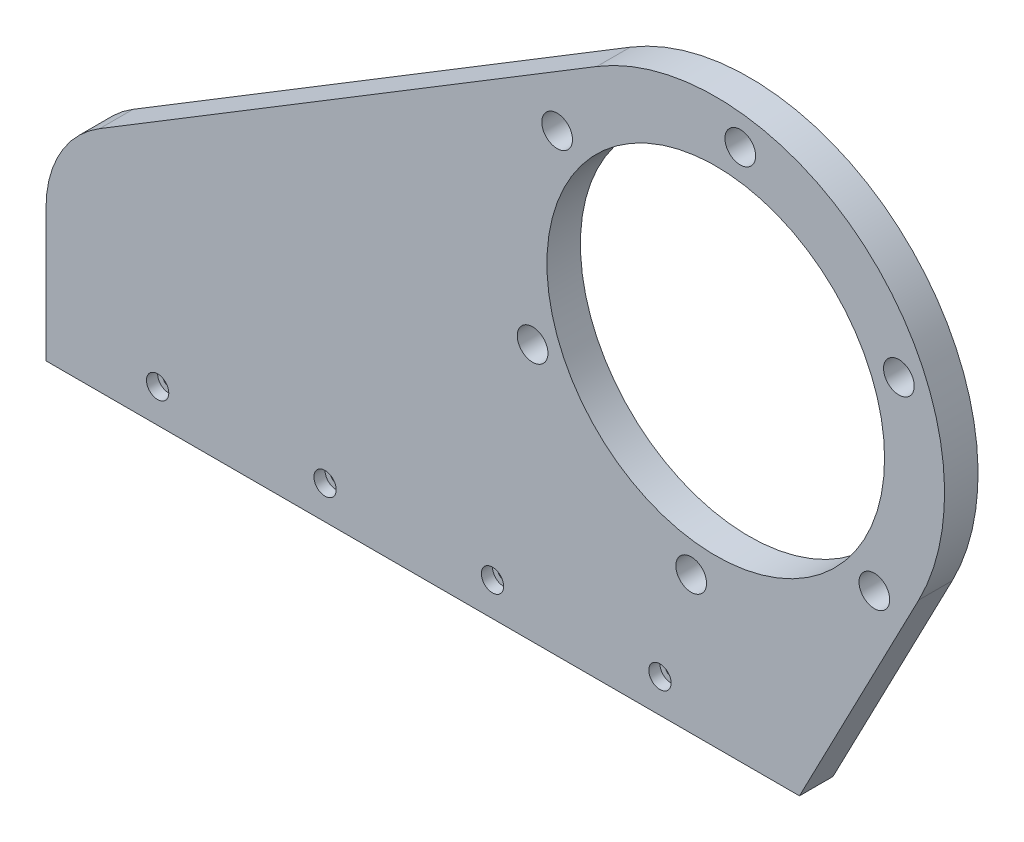
SolidWorks part; units mm, degrees
material "6061-T6 (SS)"
ref_plane "前视基准面" through (0, 0, 0) normal (0, 0, 1) x (1, 0, 0)
ref_plane "上视基准面" through (0, 0, 0) normal (0, 1, 0) x (1, 0, 0)
ref_plane "右视基准面" through (0, 0, 0) normal (1, 0, 0) x (0, 0, -1)
other "Configuration Table"
sketch "草图1" plane through (0, 0, 0) normal (0, 0, 1) x (1, 0, 0)
  line L1 (0, -120) -> (-240, -120)
  line L2 (0, -120) -> (30, -120)
  line L3 (30, -120) -> (72.7431, -37.8476)
  line L4 (-240, -120) -> (-240, -72.4885)
  line L5 (-220.7864, -38.3136) -> (-42.6122, 70.0586)
  arc A0 (72.7431, -37.8476) -> (-42.6122, 70.0586) centre (0, 0) ccw
  arc A1 (-240, -72.4885) -> (-220.7864, -38.3136) centre (-200, -72.4885) cw
  point P11 (-240, -50)
  dimension "D1" = 164
  dimension "D6" = 40
  dimension "D2" = 120
  dimension "D3" = 240
  dimension "D4" = 30
  dimension "D5" = 70
extrude "凸台-拉伸1" add sketch "草图1" along normal blind 12
sketch "草图2" plane through (0, 0, 0) normal (0, 0, 1) x (1, 0, 0)
  circle A0 centre (0, 0) radius 60.5
  dimension "D1" = 121
extrude "切除-拉伸2" cut sketch "草图2" along normal through all
sketch "草图3" plane through (0, 0, 12) normal (0, 0, 1) x (1, 0, 0)
  circle A0 centre (-200, -108) radius 2
  circle A2 centre (-140, -108) radius 2
  circle A3 centre (-80, -108) radius 2
  circle A4 centre (-20, -108) radius 2
  dimension "D3" = 4
  dimension "D1" = 4
extrude "切除-拉伸3" cut sketch "草图3" against normal through all
sketch "草图4" plane through (0, 0, 12) normal (0, 0, 1) x (1, 0, 0)
  circle A0 centre (-200, -108) radius 4
  circle A1 centre (-140, -108) radius 4
  circle A2 centre (-80, -108) radius 4
  circle A3 centre (-20, -108) radius 4
  dimension "D1" = 8
  dimension "D2" = 4
extrude "切除-拉伸4" cut sketch "草图4" against normal blind 4
sketch "草图5" plane through (0, 0, 0) normal (0, 0, -1) x (-1, 0, 0)
  circle A0 centre (20, -108) radius 4
  circle A1 centre (80, -108) radius 4
  circle A2 centre (140, -108) radius 4
  circle A3 centre (200, -108) radius 4
  dimension "D1" = 8
  dimension "D2" = 4
extrude "切除-拉伸5" cut sketch "草图5" against normal blind 4
sketch "草图6" plane through (0, 0, 0) normal (0, 0, -1) x (-1, 0, 0)
  circle A0 centre (0, 0) radius 71.25 construction
  circle A1 centre (56.8361, 42.9677) radius 5.5
  circle A3 centre (-8.793, 70.7053) radius 5.5
  circle A12 centre (65.6291, -27.7377) radius 5.5
  circle A13 centre (8.793, -70.7053) radius 5.5
  circle A14 centre (-56.8361, -42.9677) radius 5.5
  circle A15 centre (-65.6291, 27.7377) radius 5.5
  point P17 (0, 0)
  point P23 (0, 0)
  dimension "D1" = 6
  dimension "D3" = 142.5
extrude "切除-拉伸6" cut sketch "草图6" against normal through all
